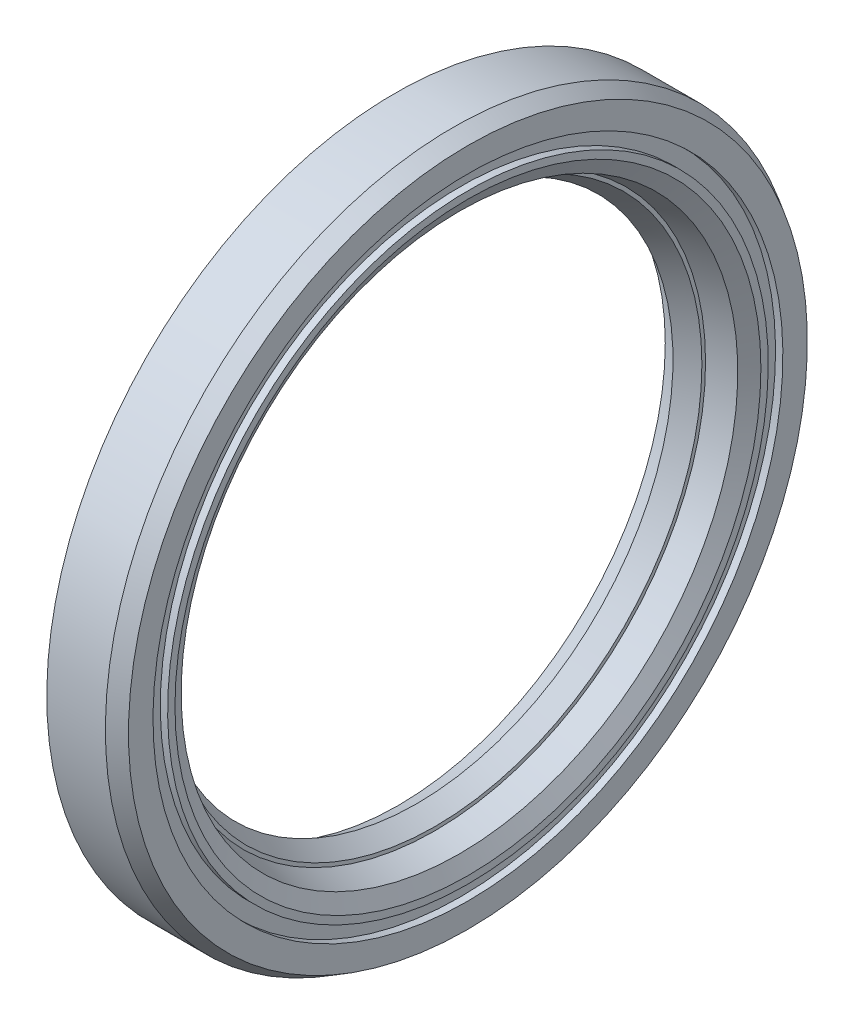
from build123d import *

# Parameters (mm, degrees)
SKETCH_1_R   = 0.8
SKETCH_1_R_2 = 0.3


with BuildPart() as part:
    # 草图1 → 旋转1 (revolve)
    with BuildSketch(Plane.XY, mode=Mode.PRIVATE) as revolve_1_sk:
        with BuildLine():
            ThreePointArc((-7.9, 39.15), (-6.85, 38.2), (-5.9, 39.25))
            Line((-5.9, 39.25), (-4.3, 39.25))
            ThreePointArc((-4.3, 39.25), (-3.734314575, 39.484314575), (-3.5, 40.05))
            Line((-3.5, 40.05), (-3.5, 43.7))
            ThreePointArc((-3.5, 43.7), (-3.734314575, 44.265685425), (-4.3, 44.5))
            Line((-4.3, 44.5), (-10, 44.5))
            Line((-10, 44.5), (-10, 47.5))
            Line((-10, 47.5), (-2, 47.5))
            Line((-2, 47.5), (0, 46.345299462))
            Line((0, 46.345299462), (0, 43))
            Line((0, 43), (-1, 43))
            Line((-1, 43), (-1, 41))
            Line((-1, 41), (0, 41))
            Line((0, 41), (0, 40))
            Line((0, 40), (-1.154700538, 38))
            Line((-1.154700538, 38), (-4.5, 36.943375673))
            Line((-4.5, 36.943375673), (-4.5, 36.443375673))
            Line((-4.5, 36.443375673), (-7, 35))
            Line((-7, 35), (-9.5, 36.443375673))
            Line((-9.5, 36.443375673), (-9.5, 39.15))
            ThreePointArc((-9.5, 39.15), (-8.7, 39.95), (-7.9, 39.15))
        make_face()
        with BuildLine():
            Line((-2.5, 41.25), (-2.5, 45))
            ThreePointArc((-2.5, 45), (-2.646446609, 45.353553391), (-3, 45.5))
            Line((-3, 45.5), (-8.5, 45.5))
            Line((-8.5, 45.5), (-8.5, 46.5))
            Line((-8.5, 46.5), (-2, 46.5))
            ThreePointArc((-2, 46.5), (-1.646446609, 46.353553391), (-1.5, 46))
            Line((-1.5, 46), (-1.5, 41.25))
            Line((-1.5, 41.25), (-2.5, 41.25))
        make_face(mode=Mode.SUBTRACT)
        with Locations((-6.9, 39.25)):
            Circle(SKETCH_1_R)
        with Locations((-6.9, 39.25)):
            Circle(SKETCH_1_R_2, mode=Mode.SUBTRACT)
    revolve(revolve_1_sk.sketch.rotate(Axis((-10, 0, 0), (1, 0, 0)), 180), axis=Axis((-10, 0, 0), (1, 0, 0)))


solid = part.part
